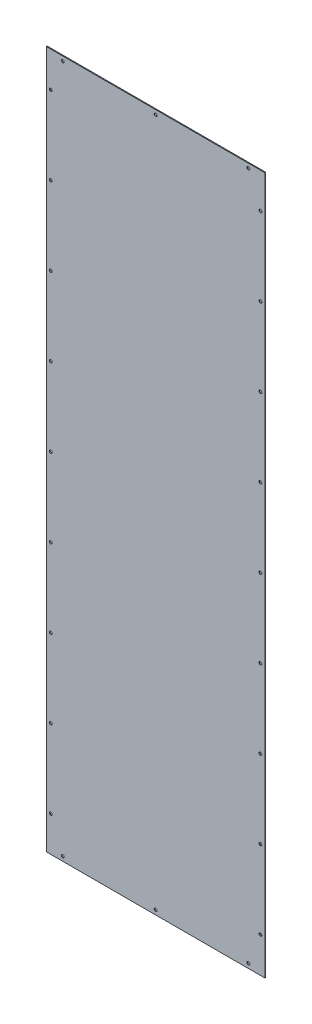
SolidWorks part; units mm, degrees
material "304"
ref_plane "前视基准面" through (0, 0, 0) normal (0, 0, 1) x (1, 0, 0)
ref_plane "上视基准面" through (0, 0, 0) normal (0, 1, 0) x (1, 0, 0)
ref_plane "右视基准面" through (0, 0, 0) normal (1, 0, 0) x (0, 0, -1)
sketch "草图1" plane through (0, 0, 0) normal (0, 0, 1) x (1, 0, 0)
  line L0 (0, 0) -> (451.2544, 0) construction
  line L1 (-247.25, 789) -> (247.25, 789)
  line L2 (-247.25, 789) -> (-247.25, -789)
  line L3 (-247.25, -789) -> (247.25, -789)
  line L4 (247.25, 789) -> (247.25, -789)
  line L5 (-247.25, 789) -> (247.25, -789) construction
  line L6 (-247.25, -789) -> (247.25, 789) construction
  line L7 (0, 0) -> (0, 412.8629) construction
  circle A0 centre (-237.25, 0) radius 3.25
  circle A1 centre (-237.25, -177.25) radius 3.25
  circle A2 centre (-237.25, -354.5) radius 3.25
  circle A3 centre (-237.25, -531.75) radius 3.25
  circle A4 centre (-237.25, -709) radius 3.25
  circle A34 centre (0, -779) radius 3.25
  circle A35 centre (0, 779) radius 3.25
  circle A36 centre (-237.25, 709) radius 3.25
  circle A37 centre (-237.25, 531.75) radius 3.25
  circle A38 centre (-237.25, 354.5) radius 3.25
  circle A39 centre (-237.25, 177.25) radius 3.25
  circle A40 centre (237.25, 177.25) radius 3.25
  circle A41 centre (237.25, 354.5) radius 3.25
  circle A42 centre (237.25, 531.75) radius 3.25
  circle A43 centre (237.25, 709) radius 3.25
  circle A44 centre (237.25, -709) radius 3.25
  circle A45 centre (237.25, -531.75) radius 3.25
  circle A46 centre (237.25, -354.5) radius 3.25
  circle A47 centre (237.25, -177.25) radius 3.25
  circle A48 centre (237.25, 0) radius 3.25
  circle A49 centre (-210, 779) radius 3.25
  circle A50 centre (210, 779) radius 3.25
  circle A51 centre (210, -779) radius 3.25
  circle A52 centre (-210, -779) radius 3.25
  point P0 (0, 0)
  dimension "D3" = 6.5
  dimension "D8" = 420
  dimension "D1" = 494.5
  dimension "D2" = 1578
  dimension "D4" = 10
  dimension "D6" = 10
  dimension "D7" = 80
  dimension "D5" = 5
extrude "凸台-拉伸1" add sketch "草图1" along normal blind 2
sketch "草图2" plane through (0, -789, 0) normal (0, -1, 0) x (1, 0, 0)
  line L0 (-247.25, 2) -> (247.25, 2) construction
  line L1 (247.25, 0) -> (244.75, 0)
  line L2 (247.25, 0) -> (247.25, 2)
  line L3 (247.25, 2) -> (244.75, 2)
  line L4 (244.75, 0) -> (244.75, 2)
  dimension "D1" = 2.5
